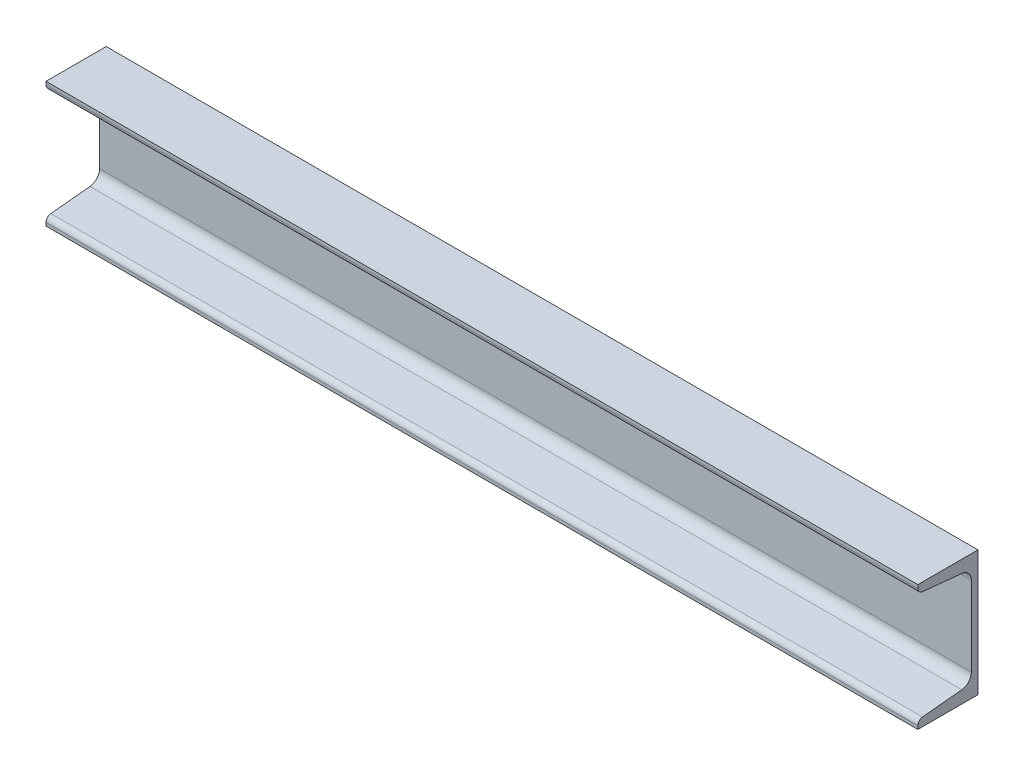
SolidWorks part; units mm, degrees
material "普通碳钢"
ref_plane "Front" through (0, 0, 0) normal (0, 0, 1) x (1, 0, 0)
ref_plane "Top" through (0, 0, 0) normal (0, 1, 0) x (1, 0, 0)
ref_plane "Right" through (0, 0, 0) normal (1, 0, 0) x (0, 0, -1)
sketch "Sketch1" plane through (0, 0, -28.2113) normal (1, 0, 0) x (0, 0, 1)
  line L0 (28.2113, -50) -> (28.2113, 50)
  line L1 (28.2113, 50) -> (76.2113, 50)
  line L2 (-69.1718, 0) -> (97.3831, 0) construction
  line L3 (33.5113, 39.365) -> (33.5113, -39.365)
  line L4 (33.5113, 39.365) -> (76.2113, 43.635)
  line L5 (76.2113, 43.635) -> (76.2113, 50)
  line L6 (33.5113, 39.365) -> (33.5113, 43.635) construction
  line L7 (33.5113, 43.635) -> (76.2113, 43.635) construction
  line L8 (54.8613, 50) -> (54.8613, 41.5) construction
  line L9 (76.2113, -43.635) -> (76.2113, -50)
  line L10 (28.2113, -50) -> (76.2113, -50)
  line L11 (33.5113, -39.365) -> (76.2113, -43.635)
  point P15 (28.2113, 0)
  point P16 (33.5113, 0)
  dimension "D1" = 21.35
  dimension "h" = 100
  dimension "b" = 48
  dimension "d" = 5.3
  dimension "t" = 8.5
  dimension "D6" = 4.27
extrude "Base" add sketch "Sketch1" along normal blind 695
fillet "Fillet1" radius 8.5 2 edges at (347.5, -39.365, 5.3) (347.5, 39.365, 5.3)
fillet "Fillet2" radius 4.25 2 edges at (347.5, -43.635, 48) (347.5, 43.635, 48)
equation "\"D1@Sketch1\" =  ( \"b@Sketch1\" - \"d@Sketch1\" )  / 2"
equation "\"D6@Sketch1\" = ( \"b@Sketch1\" - \"d@Sketch1\" )  / 10"
